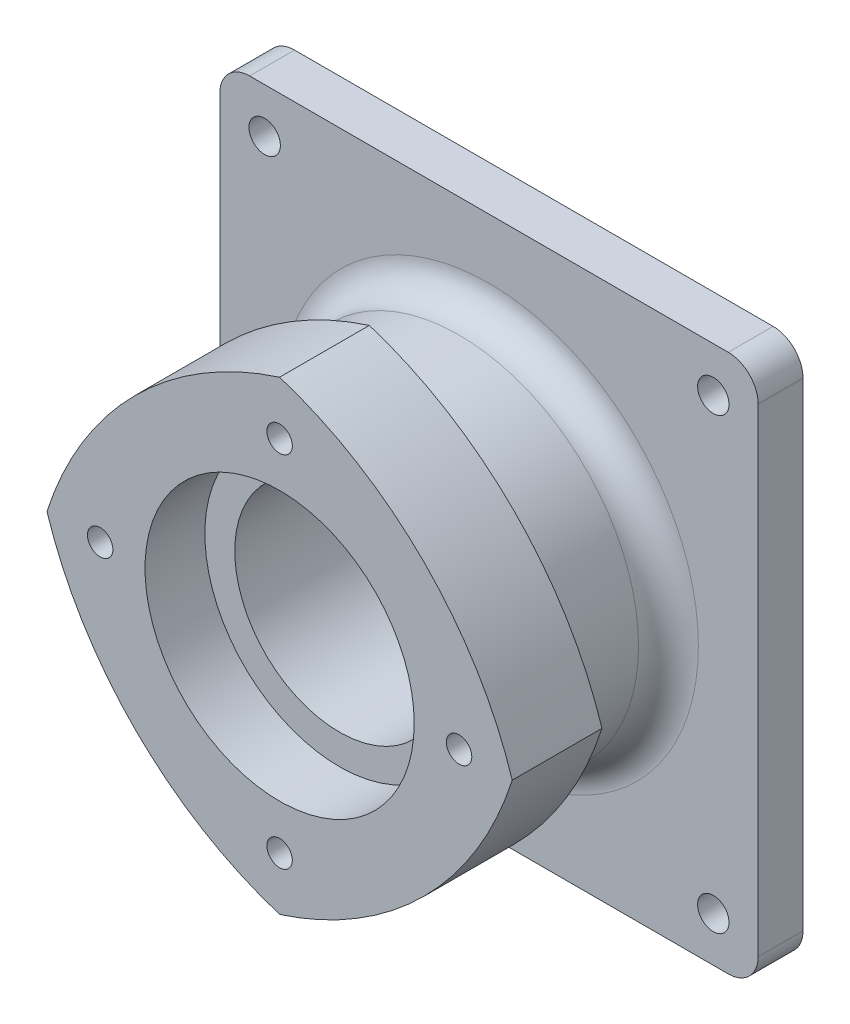
SolidWorks part; units mm, degrees
material "普通碳钢"
ref_plane "前视基准面" through (0, 0, 0) normal (0, 0, 1) x (1, 0, 0)
ref_plane "上视基准面" through (0, 0, 0) normal (0, 1, 0) x (1, 0, 0)
ref_plane "右视基准面" through (0, 0, 0) normal (1, 0, 0) x (0, 0, -1)
sketch "草图1" plane through (0, 0, 0) normal (0, 0, 1) x (1, 0, 0)
  line L1 (-80, 90) -> (80, 90)
  line L2 (-90, 80) -> (-90, -80)
  line L3 (-80, -90) -> (80, -90)
  line L4 (90, 80) -> (90, -80)
  line L5 (-90, 90) -> (90, -90) construction
  line L6 (-90, -90) -> (90, 90) construction
  line L7 (-75, -75) -> (75, -75) construction
  line L8 (-75, -75) -> (-75, 75) construction
  line L9 (-75, 75) -> (75, 75) construction
  line L10 (75, -75) -> (75, 75) construction
  line L11 (-75, -75) -> (75, 75) construction
  line L12 (-75, 75) -> (75, -75) construction
  arc A0 (-90, -80) -> (-80, -90) centre (-80, -80) ccw
  arc A1 (80, -90) -> (90, -80) centre (80, -80) ccw
  arc A2 (80, 90) -> (90, 80) centre (80, 80) cw
  arc A3 (-80, 90) -> (-90, 80) centre (-80, 80) ccw
  circle A4 centre (-75, 75) radius 5.25
  circle A5 centre (75, 75) radius 5.25
  circle A6 centre (-75, -75) radius 5.25
  circle A7 centre (75, -75) radius 5.25
  point P0 (0, 0)
  point P18 (0, 0)
  dimension "D3" = 10
  dimension "D6" = 10.5
  dimension "D1" = 180
  dimension "D2" = 180
  dimension "D4" = 150
  dimension "D5" = 150
extrude "凸台-拉伸1" add sketch "草图1" along normal blind 15
sketch "草图2" plane through (0, 0, 15) normal (0, 0, 1) x (1, 0, 0)
  circle A0 centre (0, 0) radius 60
  dimension "D1" = 120
extrude "凸台-拉伸2" add sketch "草图2" along normal blind 40
sketch "草图3" plane through (0, 0, 55) normal (0, 0, 1) x (1, 0, 0)
  line L0 (0, 77.7817) -> (77.7817, 0) construction
  line L1 (0, 77.7817) -> (-77.7817, 0) construction
  line L2 (77.7817, 0) -> (0, -77.7817) construction
  line L3 (-77.7817, 0) -> (0, -77.7817) construction
  line L4 (77.7817, 0) -> (-77.7817, 0) construction
  line L5 (0, 0) -> (142.9572, 0) construction
  arc A0 (0, 77.7817) -> (77.7817, 0) centre (-36.5246, -36.5246) cw
  arc A1 (0, 77.7817) -> (-77.7817, 0) centre (36.5246, -36.5246) ccw
  arc A2 (-77.7817, 0) -> (0, -77.7817) centre (36.5246, 36.5246) ccw
  arc A3 (0, -77.7817) -> (77.7817, 0) centre (-36.5246, 36.5246) ccw
  point P0 (0, 0)
  dimension "D4" = 120
  dimension "D5" = 120
  dimension "D6" = 120
  dimension "D7" = 120
  dimension "D1" = 110
  dimension "D2" = 110
  dimension "D3" = 45
extrude "凸台-拉伸3" add sketch "草图3" along normal blind 30
sketch "草图4" plane through (0, 0, 85) normal (0, 0, 1) x (1, 0, 0)
  line L0 (0, 0) -> (0, 127.0826) construction
  line L1 (0, 0) -> (155.9697, 0) construction
  point P3 (0, 60)
  dimension "D1" = 60
hole_wizard "M10 螺纹孔1" positions "3D草图1" profile "草图5" tap size "M10" standard "GB"
sketch3d "3D草图1"
  point P0 (0, 60, 85)
sketch "草图5" plane through (0, 60, 85) normal (1, 0, 0) x (0, -1, 0)
  line L0 (0, 0) -> (0, 24.5537)
  line L1 (0, 24.5537) -> (4.25, 22)
  line L2 (4.25, 22) -> (4.25, 0)
  line L5 (4.25, 0) -> (0, 0)
  line L10 (0, 24.5537) -> (-4.25, 22) construction
  line L11 (0, -6.35) -> (0, 107.95) construction
  dimension "螺纹孔钻头直径" = 8.5
  dimension "螺纹孔钻头深度" = 22
  dimension "导头角度" = 118
cosmetic thread "孔螺蚊线1" parameters "D1"=20, "D2"=10
pattern_circular "阵列(圆周)1" count 4 over 360 about axis through (0, 0, 0) along (0, 0, 1) of "M10 螺纹孔1"
fillet "圆角1" radius 10 1 edges at (60, 0, 15)
fillet "圆角2" radius 5 1 edges at (60, 0, 55)
sketch "草图6" plane through (0, 0, 85) normal (0, 0, 1) x (1, 0, 0)
  circle A0 centre (0, 0) radius 35
  dimension "D1" = 70
extrude "切除-拉伸1" cut sketch "草图6" against normal through all
sketch "草图7" plane through (0, 0, 85) normal (0, 0, 1) x (1, 0, 0)
  circle A0 centre (0, 0) radius 45
  dimension "D1" = 90
extrude "切除-拉伸2" cut sketch "草图7" against normal blind 20
